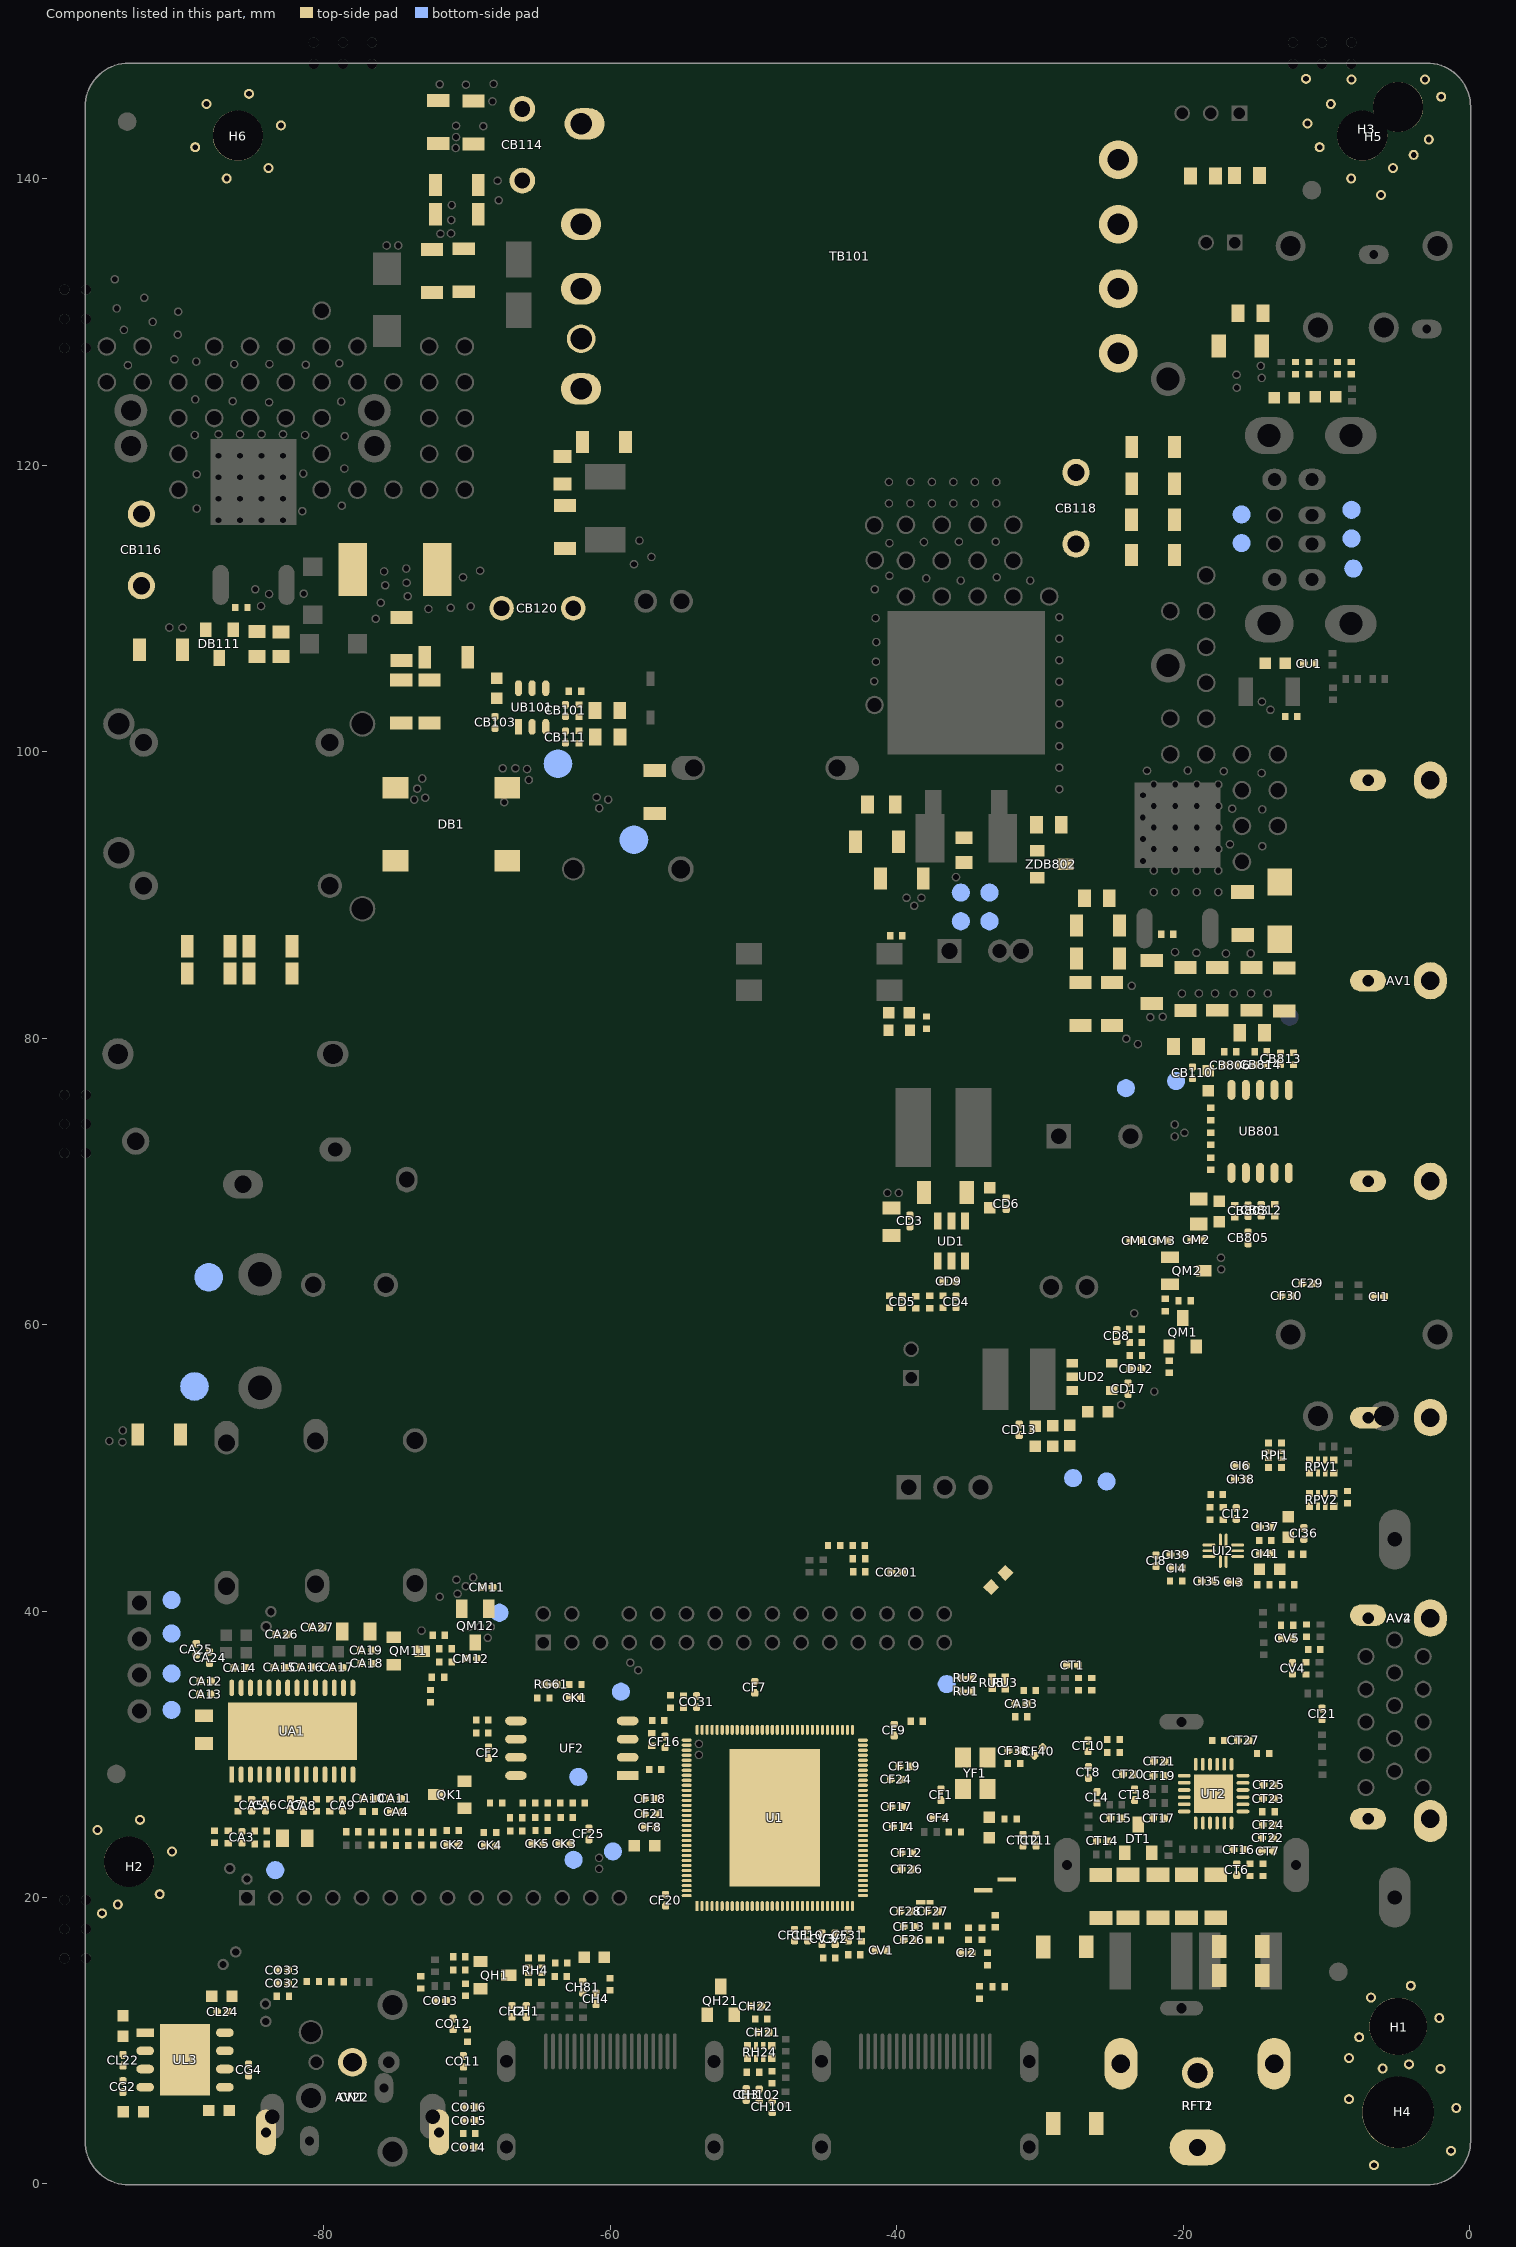
[diagram p0: the components of this part, seen from the top]
# Altium PCB MISC86372.PcbDoc (part 3 of 16)
Units mm, origin at the board's own origin, x right, y up, seen from the top; angles counter-clockwise.
Board outline 96.73 x 148.13 mm, 2 copper layers (TopLayer, BottomLayer), stack 1.571 mm thick; 578 components, 318 nets, 2702 pads, 836 vias.

## Components (designator, comment, footprint, x,y, rotation, side; value= is the part's Value field where it differs from the comment) (continued)
QK1 "General transistor,Dynatron,NPN,0.2A,40V,30-300,SOT-23,MMBT3904(f≥350MHz),BLUE ROCKET" SOT-23 -71.196,27.178 r270 top
QM1 "General transistor,Dynatron,NPN,0.2A,40V,30-300,SOT-23,MMBT3904(f≥350MHz),BLUE ROCKET" SOT-23 -20.041,59.487 r180 top
QM2 "Field-effect transistor,PMOS,-4.2A,-30V,0.052ohm@ID=-4.2A@VGS=-10V,SOT-23-3,AO3401,BLUE ROCKET" SOT-23-1 -19.726,63.762 r90 top
QM11 "General transistor,Dynatron,NPN,0.2A,40V,30-300,SOT-23,MMBT3904(f≥350MHz),BLUE ROCKET" SOT-23 -74.092,37.211 r90 top
QM12 "Field-effect transistor,PMOS,-4.3A,-30V,0.048ohm@ID=-3A@VGS=-4.5V,SOT-23-3L,NCE3407AY,NCEPOWER" SOT-23-1 -69.422,38.957 r0 top
RA1 "4K7ohm-0402-±5%-1/16W" R0402 -87.641,24.236 r270 top
RA2 "4K7ohm-0402-±5%-1/16W" R0402 -86.001,26.458 r270 top
RA3 "1Kohm-0402-±5%-1/16W" R0402 -86.672,24.222 r90 top
RA4 "NC/?" GND#2 -33.96,20.498 r180 top
RA5 "NC/?" GND#2 -32.31,21.262 r180 top
RA8 "NC/100Kohm-0402-±5%-1/16W" R0402 -84.397,24.638 r180 top
RA9 "NC/47Kohm-0402-±5%-1/16W" R0402 -84.397,23.724 r180 top
RA10 "10Kohm-0402-±1%-1/16W" R0402 -80.502,26.448 r90 top
RA11 "15Kohm-0402-±1%-1/16W" R0402 -79.588,26.448 r90 top
RA14 "1Kohm-0402-±5%-1/16W" R0402 -76.849,26.01 r0 top
RA25 "10ohm-0805-±5%-1/8W" R0805 -82.019,24.13 r180 top
RA31 "1Kohm-0402-±5%-1/16W" R0402 -9.235,126.771 r90 top
RA32 "1Kohm-0402-±5%-1/16W" R0402 -12.167,126.771 r90 top
RA33 "Thick-film resistor,RES,1/16W,180ohm,±5%,0402,SMD" R0402 -11.227,126.771 r90 top
RA34 "Thick-film resistor,RES,1/16W,180ohm,±5%,0402,SMD" R0402 -8.27,126.771 r90 top
RA35 "47Kohm-0402-±5%-1/16W" R0402 -31.318,32.614 r180 top
RA36 "10Kohm-0402-±5%-1/16W" R0402 -30.709,34.442 r0 top
RB1 "1M2ohm-1206-±5%-1/4W" R1206 -83.717,84.506 r180 top
RB2 "1M2ohm-1206-±5%-1/4W" R1206 -83.718,86.411 r180 top
RB3 "1M2ohm-1206-±5%-1/4W" R1206 -88.036,86.411 r180 top
RB4 "1M2ohm-1206-±5%-1/4W" R1206 -88.036,84.506 r180 top
RB101 "330Kohm-1206-±5%-1/4W" R1206 -74.6,103.505 r90 top
RB102 "330Kohm-1206-±5%-1/4W" R1206 -74.574,107.848 r270 top
RB103 "Thick-film resistor,RES,1/16W,2Kohm,±1%,0402,SMD" R0402 -62.189,102.845 r90 top
RB104 "NC/47Kohm-0402-±1%-1/16W" R0402 -62.189,101.016 r270 top
RB105 "Thick-film resistor,RES,1/16W,300ohm,±1%,0402,SMD" R0402 -62.465,104.216 r180 top
RB106 "68ohm-0805-±5%-1/8W" R0805 -84.658,107.516 r90 top
RB107 "20ohm-0805-±5%-1/8W" R0805 -82.982,107.49 r90 top
RB109 "10Kohm-0402-±1%-1/16W" R0402 -85.75,110.058 r180 top
RB113 "NC/150Kohm-0805-±1%-1/8W" R0805 -60.182,101.016 r0 top
RB114 "Thick-film resistor,RES,1/4W,10ohm,±5%,1206,SMD" R1206 -60.427,121.615 r0 top
RB117 "10ohm-1206-±5%-1/4W" R1206 -69.545,143.916 r90 top
RB118 "10ohm-1206-±5%-1/4W" R1206 -72.009,143.942 r90 top
RB119 "10ohm-1206-±5%-1/4W" R1206 -91.364,107.112 r180 top
RB120 "NC/10ohm-1206-±5%-1/4W" R1206 -63.17,115.67 r90 top
RB121 "Thick-film resistor,RES,1/8W,30Kohm,±1%,0805,SMD" R0805 -60.208,102.87 r180 top
RB124 "Thick-film resistor,RES,1/4W,47ohm,±5%,1206,SMD" R1206 -22.123,113.716 r180 top
RB125 "Thick-film resistor,RES,1/4W,47ohm,±5%,1206,SMD" R1206 -22.098,121.26 r180 top
RB126 "Thick-film resistor,RES,1/4W,47ohm,±5%,1206,SMD" R1206 -22.098,118.694 r180 top
RB128 "Thick-film resistor,RES,1/4W,47ohm,±5%,1206,SMD" R1206 -39.648,91.135 r0 top
RB129 "Thick-film resistor,RES,1/4W,47ohm,±5%,1206,SMD" R1206 -41.377,93.701 r0 top
RB130 "20ohm-1206-±5%-1/4W" R1206 -56.896,97.18 r90 top
RB131 "Thick-film resistor,RES,1/10W,2Kohm,±1%,0603,SMD" R0603 -39.827,80.543 r0 top
RB132 "Thick-film resistor,RES,1/16W,1.2Kohm,±1%,0402,SMD" R0402 -40.03,87.147 r0 top
RB133 "Thick-film resistor,RES,1/16W,30Kohm,±1%,0402,SMD" R0402 -18.085,74.701 r90 top
RB134 "Thick-film resistor,RES,1/16W,2Kohm,±1%,0402,SMD" R0402 -18.085,72.974 r270 top
RB135 "18Kohm-0402-±1%-1/16W" R0402 -18.085,71.222 r90 top
RB136 "Thick-film resistor,RES,1/4W,47ohm,±5%,1206,SMD" R1206 -22.123,116.18 r180 top
RB139 "NC/Thick-film resistor,RES,1/16W,51ohm,±1%,0402,SMD" R0402 -37.922,81.081 r90 top
RB140 "NC/51Kohm-0805-±1%-1/8W" R0805 -35.306,93.116 r90 top
RB141 "NC/2Mohm-1206-±5%-1/4W" R1206 -72.619,103.505 r270 top
RB142 "NC/2Mohm-1206-±5%-1/4W" R1206 -71.45,106.578 r180 top
RB143 "NC/Thick-film resistor,RES,1/4W,0ohm,±5%,1206,SMD" R1206 -91.491,52.324 r0 top
RB148 "Thick-film resistor,RES,2W,0.36ohm,±5%,2512,SMD" R2512-1 -75.032,112.7 r180 top
RB150 "Thick-film resistor,RES,1/4W,100Kohm,±5%,1206,SMD" R1206 -70.231,133.604 r90 top
RB151 "Thick-film resistor,RES,1/4W,100Kohm,±5%,1206,SMD" R1206 -72.441,133.553 r90 top
RB152 "Thick-film resistor,RES,1/4W,100Kohm,±5%,1206,SMD" R1206 -70.714,139.548 r0 top
RB153 "Thick-film resistor,RES,1/4W,100Kohm,±5%,1206,SMD" R1206 -70.715,137.516 r0 top
RB803 "Thick-film resistor,RES,1/16W,1.3Kohm,±1%,0402,SMD" R0402 -16.713,79.045 r180 top
RB804 "Thick-film resistor,RES,1/16W,20Kohm,±1%,0402,SMD" R0402 -13.614,67.97 r90 top
RB806 "Thick-film resistor,RES,1/16W,100ohm,±5%,0402,SMD" R0402 -16.408,67.92 r90 top
RB807 "Thick-film resistor,RES,1/8W,10ohm,±5%,0805,SMD" R0805 -26.033,89.764 r0 top
RB808 "10Kohm-0402-±1%-1/16W" R0402 -21.107,87.249 r0 top
RB813 "Thick-film resistor,RES,1/16W,100ohm,±5%,0402,SMD" R0402 -12.294,78.562 r270 top
RB814 "Thick-film resistor,RES,1/8W,510Kohm,±1%,0805-Auto,SMD" R0805 -19.812,79.4 r0 top
RB816 "33ohm-0805-±5%-1/8W" R0805 -18.923,67.894 r90 top
RB818 "Thick-film resistor,RES,1/4W,2ohm,±1%,1206,SMD" R1206 -12.954,83.388 r270 top
RB819 "Thick-film resistor,RES,1/4W,2ohm,±1%,1206,SMD" R1206 -17.628,83.439 r270 top
RB820 "Thick-film resistor,RES,1/4W,2ohm,±1%,1206,SMD" R1206 -15.24,83.439 r270 top
RB821 "Thick-film resistor,RES,1/4W,2ohm,±1%,1206,SMD" R1206 -25.959,85.547 r180 top
RB822 "Thick-film resistor,RES,1/4W,2ohm,±1%,1206,SMD" R1206 -25.959,87.859 r180 top
RB823 "Thick-film resistor,RES,1/4W,2ohm,±1%,1206,SMD" R1206 -22.2,83.922 r270 top
RB824 "Thick-film resistor,RES,1/4W,2.4ohm,±5%,1206,SMD" R1206 -19.837,83.414 r270 top
RB825 "Thick-film resistor,RES,1/4W,51Kohm,±1%,1206,SMD" R1206 -24.968,82.372 r270 top
RB826 "Thick-film resistor,RES,1/4W,51Kohm,±1%,1206,SMD" R1206 -27.178,82.372 r270 top
RB833 "Thick-film resistor,RES,1/16W,40.2Kohm,±1%,0402,SMD" R0402 -14.58,79.045 r0 top
RB834 "Thick-film resistor,RES,1/8W,200Kohm,±1%,0805,SMD" R0805 -15.189,80.366 r180 top
RB835 "NC/Thick-film resistor,RES,1/8W,330Kohm,±1%,0805,SMD" R0805 -29.385,94.894 r180 top
RB845 "0ohm-0805-±5%-1/8W" R0805 -18.618,140.183 r0 top
RB846 "NC/0ohm-0805-±5%-1/8W" R0805 -15.545,140.208 r0 top
RB847 "0ohm-0805-±5%-1/8W" R0805 -15.309,130.607 r180 top
RD1 "100Kohm-0402-±5%-1/16W" R0402 -36.779,61.582 r90 top
RD3 "Thick-film resistor,RES,1/16W,33Kohm,±1%,0402,SMD" R0402 -38.677,61.564 r270 top
RD5 "Thick-film resistor,RES,1/16W,6.04Kohm,±1%,0402,SMD" R0402 -40.513,61.589 r90 top
RD6 "NC/?" R0402 -37.694,61.57 r270 top
RD7 "Thick-film resistor,RES,1/16W,100Kohm,±5%,0402,SMD" R0402 -23.333,59.675 r0 top
RD8 "Thick-film resistor,RES,1/16W,13Kohm,±1%,0402,SMD" R0402 -23.317,58.75 r0 top
RD9 "Thick-film resistor,RES,1/16W,12Kohm,±1%,0402,SMD" R0402 -23.305,57.83 r180 top
RF3 "NC/4K7ohm-0402-±5%-1/16W" R0402 -56.865,28.931 r180 top
RF8 "NC/4K7ohm-0402-±5%-1/16W" R0402 -42.647,44.564 r180 top
RF9 "NC/4K7ohm-0402-±5%-1/16W" R0402 -44.374,44.564 r0 top
RF10 "NC/100ohm-0402-±5%-1/16W" R0402 -42.639,43.649 r0 top
RF11 "NC/100ohm-0402-±5%-1/16W" R0402 -42.621,42.739 r0 top
RF12 "68ohm-0402-±5%-1/16W" R0402 -37.338,17.043 r0 top
RF13 "4K7ohm-0402-±5%-1/16W" R0402 -62.433,34.87 r0 top
RF16 "68ohm-0402-±5%-1/16W" R0402 -42.469,17.374 r90 top
RF23 "4K7ohm-0402-±5%-1/16W" R0402 -57.099,31.029 r90 top
RF24 "1Kohm-0402-±5%-1/16W" R0402 -31.814,29.352 r180 top
RF29 "4K7ohm-0402-±5%-1/16W" R0402 -56.642,32.36 r180 top
RF43 "4K7ohm-0402-±5%-1/16W" R0402 -27.305,34.9 r270 top
RF44 "4K7ohm-0402-±5%-1/16W" R0402 -26.391,34.9 r270 top
RFT1 "NC/RF jack,RF JACK,H,IEC,T14.5,CH6.3,12.4×13.2×7.7mm,DIP,LHD-020 assembly,LHD" ANT-IEC14.5-H-4 -19,2.3 r0 top locked
RFT2 "RF jack,RF JACK,H,F,T14.5,CH6.3,without pipe,12.4×13.2×7.7mm,DIP,LHD" T-13.2×12.4×7.7-F14.5 -19,2.3 r0 top locked
RG61 "NC/" R0402SC -64.135,34.87 r180 top
RH3 "1Kohm-0402-±5%-1/16W" R0402 -70.104,13.564 r270 top
RH4 "Resistor array,RES ARRAY,1/16W,4×10Kohm,±5%,0402,SMD" RA0402 -65.253,14.935 r0 top
RH5 "33ohm-0402-±5%-1/16W" R0402 -63.43,15.418 r0 top
RH6 "33ohm-0402-±5%-1/16W" R0402 -63.449,14.494 r0 top
RH23 "1Kohm-0402-±5%-1/16W" R0402 -49.463,11.527 r180 top
RH24 "Resistor array,RES ARRAY,1/16W,4×10Kohm,±5%,0402,SMD" RA0402 -49.58,9.199 r90 top
RH25 "33ohm-0402-±5%-1/16W" R0402 -50.038,7.798 r180 top
RH26 "33ohm-0402-±5%-1/16W" R0402 -48.717,7.442 r270 top
RH81 "22Kohm-0402-±5%-1/16W" R0402 -70.536,14.935 r0 top
RH82 "33Kohm-0402-±5%-1/16W" R0402 -70.536,15.861 r0 top
RH83 "100ohm-0402-±5%-1/16W" R0402 -60.02,13.938 r270 top
RH102 "Thick-film resistor,RES,1/16W,1.2Kohm,±1%,0402,SMD" R0402 -63.043,25.578 r0 top
RH103 "220ohm-0402-±5%-1/16W" R0402 -63.932,26.594 r180 top
RH104 "4K7ohm-0402-±5%-1/16W" R0402 -68.936,31.487 r0 top
RH105 "220ohm-0402-±5%-1/16W" R0402 -62.205,26.594 r180 top
RH106 "4K7ohm-0402-±5%-1/16W" R0402 -68.936,32.401 r0 top
RI1 "75ohm-0402-±5%-1/16W" R0402 -33.122,18.339 r90 top
RI2 "33ohm-0402-±5%-1/16W" R0402 -35,17.478 r90 top
RI3 "NC/1Kohm-0402-±5%-1/16W" R0402 -20.498,42.088 r0 top
RI4 "0ohm-0402-±5%-1/16W" R0402 -8.534,47.955 r90 top
RI5 "NC/0ohm-0402-±5%-1/16W" R0402 -16.472,41.993 r180 top
RI6 "NC/0ohm-0402-±5%-1/16W" R0402 -20.496,42.996 r180 top
RI37 "NC/200Kohm-0402-±5%-1/16W" R0402 -14.275,44.929 r0 top
RI38 "NC/200Kohm-0402-±5%-1/16W" R0402 -17.213,46.805 r90 top
RI39 "NC/200Kohm-0402-±5%-1/16W" R0402 -17.653,48.133 r180 top
RI40 "NC/200Kohm-0402-±5%-1/16W" R0402 -18.127,46.805 r90 top
RI42 "NC/1Kohm-0402-±5%-1/16W" R0402 -12.675,41.834 r0 top
RI43 "NC/1Kohm-0402-±5%-1/16W" R0402 -12.04,43.967 r0 top
RI48 "NC/100ohm-0402-±5%-1/16W" R0402 -14.402,41.834 r0 top
RK1 "4K7ohm-0402-±5%-1/16W" R0402 -67.97,26.594 r180 top
RK2 "1Kohm-0402-±5%-1/16W" R0402 -64.668,33.925 r0 top
RK3 "4K7ohm-0402-±1%-1/16W" R0402 -66.575,25.569 r180 top
RK4 "1Kohm-0402-±5%-1/16W" R0402 -64.808,25.585 r180 top
RK5 "22ohm-0402-±5%-1/16W" R0402 -70.993,24.669 r0 top
RK6 "510ohm-0402-±1%-1/16W" R0402 -78.008,24.595 r0 top
RK7 "680ohm-0402-±1%-1/16W" R0402 -72.782,23.663 r0 top
RK8 "1Kohm-0402-±1%-1/16W" R0402 -72.791,24.559 r0 top
RK9 "1K2ohm-0402-±1%-1/16W" R0402 -74.535,24.567 r0 top
RK10 "1Kohm-0402-±5%-1/16W" R0402 -68.395,24.544 r180 top
RK11 "2K2ohm-0402-±1%-1/16W" R0402 -74.534,23.641 r0 top
RK12 "4K7ohm-0402-±1%-1/16W" R0402 -76.246,23.658 r0 top
RK13 "33Kohm-0402-±5%-1/16W" R0402 -65.679,26.594 r180 top
RK14 "510ohm-0402-±1%-1/16W" R0402 -64.795,24.666 r0 top
RK15 "10Kohm-0402-±5%-1/16W" R0402 -66.573,24.648 r0 top
RK16 "15Kohm-0402-±1%-1/16W" R0402 -76.275,24.573 r0 top
RM1 "10Kohm-0402-±5%-1/16W" R0402 -38.608,32.309 r180 top
RM2 "4K7ohm-0402-±5%-1/16W" R0402 -20.98,57.048 r90 top
RM3 "4K7ohm-0402-±5%-1/16W" R0402 -21.252,61.366 r90 top
RM4 "Thick-film resistor,RES,1/16W,100Kohm,±5%,0402,SMD" R0402 -19.906,61.663 r180 top
RM11 "4K7ohm-0402-±5%-1/16W" R0402 -72.028,35.377 r180 top
RM12 "10Kohm-0402-±5%-1/16W" R0402 -72.542,34.061 r270 top
RM13 "4K7ohm-0402-±5%-1/16W" R0402 -71.975,38.303 r180 top
RM14 "47Kohm-0402-±5%-1/16W" R0402 -71.501,36.452 r0 top
RM15 "NC/4K7ohm-0402-±5%-1/16W" R0402 -71.501,37.363 r180 top
RO1 "NC/75ohm-0402-±5%-1/16W" R0402 -36.855,18.009 r180 top
RO2 "NC/0ohm-0402-±5%-1/16W" R0402 -73.228,14.072 r90 top
RO3 "NC/0ohm-0402-±5%-1/16W" R0402 -80.762,14.129 r0 top
RO4 "NC/0ohm-0402-±5%-1/16W" R0402 -79.045,14.118 r180 top
RO12 "NC/510ohm-0402-±1%-1/16W" R0402 -69.977,10.363 r270 top
RO15 "NC/510ohm-0402-±1%-1/16W" R0402 -69.85,3.516 r0 top
RO21 "Thick-film resistor,RES,1/16W,150ohm,±1%,0402,SMD" R0402 -54.89,33.674 r270 top
RO22 "75ohm-0402-±5%-1/16W" R0402 -55.804,33.68 r270 top
RO33 "NC/0ohm-0402-±5%-1/16W" R0402 -82.855,13.106 r0 top
ROUT+ "DM0" TP -90.627,40.767 r180 bottom
ROUT- "DM0" TP -90.627,38.43 r180 bottom
RPI1 "Resistor array,RES ARRAY,1/16W,4×10Kohm,±5%,0402,SMD" RA0402 -13.589,50.876 r180 top
RPV1 "NC/Resistor array,RES ARRAY,1/16W,4×10Kohm,±5%,0402,SMD" RA0402 -10.342,50.082 r270 top
RPV2 "NC/Resistor array,RES ARRAY,1/16W,4×10Kohm,±5%,0402,SMD" RA0402 -10.342,47.759 r90 top
RT1 "Ferrite bead,BEAD,300ohm,0402,800mA,SMD,TP,FCM1005KF-301T08" R0402 -35.941,24.566 r180 top
RT2 "22ohm-0402-±5%-1/16W" R0402 -15.345,21.924 r90 top
RT3 "22ohm-0402-±5%-1/16W" R0402 -14.43,21.924 r90 top
RT4 "0ohm-0402-±5%-1/16W" R0402 -24.867,30.124 r180 top
RT5 "0ohm-0402-±5%-1/16W" R0402 -24.867,31.039 r180 top
RT6 "1K8ohm-0402-±5%-1/16W" R0402 -14.049,25.988 r180 top
RT7 "10Kohm-0402-±5%-1/16W" R0402 -32.055,25.476 r0 top
RT8 "100ohm-0402-±5%-1/16W" R0402 -17.551,30.963 r180 top
RU1 "NC/0ohm-0402-PCB" R0402SC -35.149,34.413 r0 top
RU2 "NC/0ohm-0402-PCB" R0402SC -35.149,35.327 r0 top
RU3 "NC/0ohm-0402-PCB" R0402SC -32.423,34.976 r90 top
RU4 "0ohm-0402-±5%-1/16W" R0402 -12.464,102.457 r180 top
RU5 "NC/0ohm-0402-PCB" R0402SC -33.335,34.99 r90 top
RV1 "75ohm-0402-±5%-1/16W" R0402 -34.043,17.478 r270 top
RV2 "33ohm-0402-±5%-1/16W" R0402 -33.655,15.705 r270 top
RV3 "75ohm-0402-±5%-1/16W" R0402 -32.893,13.767 r180 top
RV4 "33ohm-0402-±5%-1/16W" R0402 -42.977,16.002 r180 top
RV5 "75ohm-0402-±5%-1/16W" R0402 -34.214,13.368 r90 top
RV6 "NC/10Kohm-0402-±5%-1/16W" R0402 -11.43,35.992 r90 top
RV7 "NC/100ohm-0402-±5%-1/16W" R0402 -10.846,37.313 r180 top
RV8 "NC/10Kohm-0402-±5%-1/16W" R0402 -11.396,38.633 r90 top
RV9 "NC/100ohm-0402-±5%-1/16W" R0402 -12.751,39.012 r180 top
RV10 "33ohm-0402-±5%-1/16W" R0402 -44.704,15.773 r180 top
RXD "" TP -62.23,28.423 r90 bottom
S/N1 "Barcode" Barcode -17.704,58.953 r270 bottom
TB101 "Transformer,EQ2414,300uH,0.2×1P,26Ts,H14.5MAX,SYEQ2414Z-T012064B(BLACK),DIP,SQ" T/EQ2414*10 -40.538,134.569 r0 top
TP-TDT "" TP-TDT -61,96.5 r135 bottom
TP_12VA+ "NC/" TP -35.527,90.154 r180 bottom
TP_12VA- "NC/" TP -33.527,90.154 r180 bottom
TP_12VB+ "NC/" TP -35.527,88.154 r180 bottom
TP_12VB- "NC/" TP -33.527,88.154 r180 bottom
TP_L "NC/" TP-80 -88.036,63.297 r180 bottom
TP_LED+ "NC/" TP -20.5,77 r180 bottom
TP_LED- "NC/" TP -24,76.5 r180 bottom
TP_N "NC/" TP-80 -89.027,55.677 r180 bottom
TXD "" TP -62.56,22.631 r180 bottom
U1 "TV main chip,IC Main Chip,MSD3553ZW-005X,32bit,Single-Core,QFN128,SMD,MTK" QFN128/0.35-1-9 -48.513,25.556 r90 top locked
UA1 "Audio amplifier,IC Audio AMP,Class D,2×10W@13.0V@8ohm,HTSSOP-28,SMD,RDA3118E28B,RDA" SSOP28/0.65-5 -82.197,31.611 r90 top
UART_RX "DM0" TP -27.686,49.276 r90 bottom
UART_TX "DM0" TP -25.349,49.047 r90 bottom
UB101 "PWM controller,IC PWM Controller,100KHZ,SOT23-6,SMD,LD5537B3GL,Leadtrend" SOT-26 -65.456,103.077 r180 top
UB801 "PWM controller,IC PWM Controller,10KHz-1MHz,SSOP10,SMD,SY7710FHC,silergy" SOP10/1.0-1 -14.63,73.482 r90 top
UD1 "DC-DC converter,IC DCDC,Syn,2A,18V,500KHz,SOT23-6,SMD,LC2332CB6TR,Leadchip" SOT-23-6 -36.189,65.831 r180 top
UD2 "DC-DC converter,IC DCDC,Syn,1.2A,6.0V,1.5MHz,SOT23-5,SMD,TMI3408,TOLL" SOT-23-5 -26.365,56.343 r270 top locked
UF2 "SPI FLASH chip,IC SPI FLASH,4MB,32Mb,SOIC8,SMD,W25Q32JVSSIQ,Winbond" SOIC8 -62.687,30.42 r180 top locked
UI2 "NC/AZAW2213F" QFN10/0.4 -17.206,44.208 r270 top
UL3 "LDO regulator,IC LDO,1A,3.3V,12V,ESOP-8,SMD,LC1118CS8TR1833,Leadchip" SOP8/1.27-3 -89.689,8.66 r0 top
UT2 "Silicon RF tuner,IC Si Tuner,QFN24,SMD,R842,Rafael" QFN24/0.5-3 -17.882,27.254 r90 top
VCC_PANEL "TEST" TP -67.742,39.878 r270 bottom
VDDC_CORE "TEST" TP -36.513,34.9 r0 bottom
XXXXXX "PCB_TIME" PCB_TIME -19.845,45.677 r180 top
XXXXXXXXXXXXXX "PCB_NAME" PCB_NAME -18.721,38.285 r180 top
YF1 "Passive crystal,SPXO,24MHz,±10ppm,12pF,SMD3225,SMD,2.3.3.240001234,MDH" XTAL-S-3 -34.519,28.677 r270 top
ZDB801 "TVS diode,DIO ESD,121V,SMA,SMD,SMAJ75A,YJ" DIODE-SMA-1 -13.259,88.9 r90 top
ZDB802 "Zener diode,DIO ZEN,5.6V,350mW,SOT-23,SMD,BZX84C5V6,KEXIN" SO-23 -29.185,92.138 r90 top
用于U1 "NC/Glue, 0.1g, silicone" "Heat-Shrinkable Tube" -44.936,29.365 r90 top

## Footprints (in the part's own frame and the unit in brackets; to place one, negate y for a bottom-side part, rotate by r counter-clockwise, add the part's x,y. Pads: shape width x height; smd on the part's side, far side on the other; paste and mask are expansions set on the pad)
AI_GRIPPER_V [mm] "3D shape for vertical type AI equipment  (AI爪子)"
  round 1.5 on Mech5: 0(0,-2.5) 1(0,0) 2(0,2.5)
  body extent -29.13,-4.7 2.5,4.7, height 54.74
ANT-IEC14.5-H-4 [mm] "联宏达；13.2×12.4×7.7mm LHD-020 中心高度6.3mm 160323(18.03.09更新脚距）,向内扩宽丝印,0703_2018（18.08.29 更新短槽孔）"
  oval 2.5x3.8 on Top Overlay paste-4 mask-4: 0(-5.35,6.1) 0(5.35,6.1)
  oval 4.1x2.7 on Top Overlay paste-4 mask-4: 0(0,0.25)
  round 2.4 on Top Overlay: 0(0,5.45)
  round 2.2 hole 1.4: 1(0,5.45)
  oval 2.3x3.6 hole 1.3 slot 2.6 at 90 deg: 2(-5.35,6.1) 4(5.35,6.1)
  oval 3.9x2.5 hole 1.2 slot 2.6 at 0 deg: 3(0,0.25)
  KeepOutLayer pour cut-out: 0,3.95 -0.574,4.064 -1.061,4.389 -1.386,4.876 -1.5,5.45 -1.5,5.45 -1.386,6.024 -1.061,6.511 -0.574,6.836 0,6.95 0,6.95 0.574,6.836 1.061,6.511 1.386,6.024 1.5,5.45 1.5,5.45 1.386,4.876 1.061,4.389 0.574,4.064 0,3.95
  silkscreen extent -6.3,0 6.3,7.9, body extent -7.55,-35.2 7.55,7.7, height 13.76
ASSE3.5C-3#1 [mm] "定位孔(顶底层上锡) (18.11.28 切换为扇形paste）"
  round 3.5 hole 3.5 unplated mask+0: 0(0,0)
  round 0.7 hole 0.4: 1(-0.778,-2.994) 2(-1.881,-3.602) 3(-2.195,2.213) 4(0.774,2.919) 5(3.005,0.716) 6(2.143,-2.266)
  KeepOutLayer pour cut-out: 0,-2.05 -0.785,-1.894 -1.45,-1.45 -1.894,-0.785 -2.05,0 -2.05,0 -1.894,0.785 -1.45,1.45 -0.785,1.894 0,2.05 0,2.05 0.785,1.894 1.45,1.45 1.894,0.785 2.05,0 2.05,0 1.894,-0.785 1.45,-1.45 0.785,-1.894 0,-2.05
ASSE3.5C-3#2 [mm] "定位孔(顶底层上锡) (18.11.28 切换为扇形paste）"
  round 3.5 hole 3.5 unplated mask+0: 0(0,0)
  round 0.7 hole 0.4: 1(-0.778,-2.994) 2(-2.979,-0.807) 3(-2.195,2.213) 4(-0.757,3.914) 5(3.588,-1.344) 6(2.143,-2.266)
  KeepOutLayer pour cut-out: 0,-2.05 -0.785,-1.894 -1.45,-1.45 -1.894,-0.785 -2.05,0 -2.05,0 -1.894,0.785 -1.45,1.45 -0.785,1.894 0,2.05 0,2.05 0.785,1.894 1.45,1.45 1.894,0.785 2.05,0 2.05,0 1.894,-0.785 1.45,-1.45 0.785,-1.894 0,-2.05
ASSE3.5C-3#3 [mm] "定位孔(顶底层上锡) (18.11.28 切换为扇形paste）"
  round 3.5 hole 3.5 unplated mask+0: 0(0,0)
  round 0.7 hole 0.4: 1(-1.198,-6.138) 2(-6.331,-1.156) 3(-6.43,1.964) 4(1.876,1.914) 5(3.005,0.716) 6(2.143,-2.266)
  KeepOutLayer pour cut-out: 0,-2.05 -0.785,-1.894 -1.45,-1.45 -1.894,-0.785 -2.05,0 -2.05,0 -1.894,0.785 -1.45,1.45 -0.785,1.894 0,2.05 0,2.05 0.785,1.894 1.45,1.45 1.894,0.785 2.05,0 2.05,0 1.894,-0.785 1.45,-1.45 0.785,-1.894 0,-2.05
ASSE3.5C-3#4 [mm] "定位孔(顶底层上锡) (18.11.28 切换为扇形paste）"
  round 3.5 hole 3.5 unplated mask+0: 0(0,0)
  round 0.7 hole 0.4: 1(-0.778,-2.994) 2(-2.979,-0.807) 3(-2.195,2.213) 4(0.774,2.919) 5(3.005,0.716) 6(2.143,-2.266)
  KeepOutLayer pour cut-out: 0,-2.05 -0.785,-1.894 -1.45,-1.45 -1.894,-0.785 -2.05,0 -2.05,0 -1.894,0.785 -1.45,1.45 -0.785,1.894 0,2.05 0,2.05 0.785,1.894 1.45,1.45 1.894,0.785 2.05,0 2.05,0 1.894,-0.785 1.45,-1.45 0.785,-1.894 0,-2.05
ASSE4.0C-3 [mm] "定位孔(顶底层上锡)(17.12.09更新过孔位置）18.11.22 更新paste形状为扇形。"
  round 4 hole 4 unplated mask+0: 0(0,0)
  round 0.7 hole 0.4: 1(-2.72,-0.754) 2(-1.893,2.011) 3(0.891,2.84) 4(2.873,0.584) 5(0.758,-2.643) 6(-1.075,-2.937)
  KeepOutLayer pour cut-out: 0,-2.3 -0.88,-2.125 -1.626,-1.626 -2.125,-0.88 -2.3,0 -2.3,0 -2.125,0.88 -1.626,1.626 -0.88,2.125 0,2.3 0,2.3 0.88,2.125 1.626,1.626 2.125,0.88 2.3,0 2.3,0 2.125,-0.88 1.626,-1.626 0.88,-2.125 0,-2.3
ASSE5.0C-3 [mm] "定位孔(顶底层上锡) (18.12.13更新）"
  round 5 hole 5 unplated mask+0: 0(0,0)
  round 0.7 hole 0.4: 1(-3.423,3.787) 2(-3.432,0.923) 3(-1.678,-3.689) 4(3.691,-2.689) 5(4.06,0.309) 6(2.958,3.038)
  KeepOutLayer pour cut-out: 0,-2.8 -1.072,-2.587 -1.98,-1.98 -2.587,-1.072 -2.8,0 -2.8,0 -2.587,1.072 -1.98,1.98 -1.072,2.587 0,2.8 0,2.8 1.072,2.587 1.98,1.98 2.587,1.072 2.8,0 2.8,0 2.587,-1.072 1.98,-1.98 1.072,-2.587 0,-2.8
AV1-H-4 [mm] "强生；AV38A-01S-5020;中心高度为5.5mm;14.08.09;170502更新信号脚孔径;170902更新接地脚宽度,17.12.29更新接地脚孔长度（18.05.07 更新地脚孔长?"
  round 2 hole 1.3 mask+0.076: 1(0,8.05)
  round 2.2 on Top Overlay mask+0.076: 2(0,8.05)
  oval 1.4x3.2 hole 0.7 slot 2.5 at 90 deg mask+0.076: 2(6.05,3.15) 3(-6.05,3.15)
  oval 1.6x3.4 on Top Overlay mask+0.076: 3(-6.05,3.15) 3(6.05,3.15)
  silkscreen extent -6.4,0 6.4,8.7, body extent -7.25,-51.37 7.25,8.55, height 12.75
AV3-H14-15#1 [mm] "宇球；RC075-F03L3BY-A; 中心高度：5.5mm;15.11.24;170401兼容物料，更新高度;170802加大接地脚焊盘（18.03.09更新孔距）"
  oval 2.8x2.5 on Top Overlay: 0(-14,2.75) 0(0,2.75) 0(14,2.75)
  oval 1.7x2.7 on Top Overlay: 0(-14,7.1) 0(0,7.1) 0(14,7.1)
  oval 1.5x2.5 hole 0.8 slot 1.8 at 90 deg: 1(-14,7.1) 3(0,7.1) 5(14,7.1)
  oval 2.6x2.3 hole 1.3 slot 1.6 at 0 deg: 2(-14,2.75) 4(0,2.75) 6(14,2.75)
  silkscreen extent -20.3,0 20.3,7.8, body extent -20.1,-9 20.1,7.9, height 10.7
AV3-H14-15#2 [mm] "宇球；RC075-F03L3BY-A; 中心高度：5.5mm;15.11.24;170401兼容物料，更新高度;170802加大接地脚焊盘（18.03.09更新孔距）"
  oval 2.8x2.5 on Top Overlay: 0(-14,2.75) 0(0,2.75) 0(14,2.75)
  oval 1.7x2.7 on Top Overlay: 0(-14,7.1) 0(0,7.1) 0(14,7.1)
  oval 1.5x2.5 hole 0.8 slot 1.8 at 90 deg: 1(-14,7.1) 5(14,7.1)
  oval 2.6x2.3 hole 1.3 slot 1.6 at 0 deg: 2(-14,2.75) 4(0,2.75) 6(14,2.75)
  oval 1.5x2.5 hole 0.8 slot 1.8 at 90 deg copper offset 0.2,0: 3(0,7.1)
  silkscreen extent -20.3,0 20.3,7.8, body extent -20.1,-9 20.1,7.9, height 10.7
AV3-H14-15#3 [mm] "宇球；RC075-F03L3BY-A; 中心高度：5.5mm;15.11.24;170401兼容物料，更新高度;170802加大接地脚焊盘（18.03.09更新孔距）"
  oval 2.8x2.5 on Top Overlay: 0(-14,2.75) 0(0,2.75) 0(14,2.75)
  oval 1.7x2.7 on Top Overlay: 0(-14,7.1) 0(0,7.1) 0(14,7.1)
  oval 1.5x2.5 hole 0.8 slot 1.8 at 90 deg: 1(-14,7.1) 5(14,7.1)
  oval 2.6x2.3 hole 1.3 slot 1.6 at 0 deg copper offset -0.32,0: 2(-14,2.75)
  oval 1.5x2.5 hole 0.8 slot 1.8 at 90 deg copper offset 0.2,0: 3(0,7.1)
  oval 2.6x2.3 hole 1.3 slot 1.6 at 0 deg: 4(0,2.75) 6(14,2.75)
  silkscreen extent -20.3,0 20.3,7.8, body extent -20.1,-9 20.1,7.9, height 10.7
B/YBS3010A [mm] "YJ,YBS3010A,18.04.17"
  rect 1.5x1.8 smd: 1(2.55,3.9) 2(2.55,-3.9) 3(-2.55,-3.9) 4(-2.55,3.9)
  silkscreen extent -3.35,-3.7 3.35,5.74, body extent -3.35,-3.7 3.35,3.7, height 1.5
Barcode [mm] "(18.12.17 更新为白油）"
  round 0.3 on Mech2: 0(0,0)
  silkscreen extent -15,-4 15,4
C0402 [mm] "片式电容  2018.10.7 替换为兼容0201封装"
  rrect50% 0.45x0.5 smd mask+0.051: 1(-0.425,0) 2(0.425,0)
  rect 0.3x0.3 smd mask+0.051: 1(-0.25,0) 2(0.25,0)
  rect 0.6x0.6 on Top Solder: 2(0,0)
  TopLayer pour cut-out: -0.318,0.302 -0.318,-0.303 0.306,-0.303 0.306,0.302
  silkscreen extent -0.88,-0.4 0.88,0.4, body extent -0.5,-0.25 0.5,0.25, height 0.5
C0603 [mm] "片式电容"
  rect 0.8x0.8 smd mask+0.076: 1(-0.706,0) 2(0.706,0)
  silkscreen extent -1.39,-0.55 1.39,0.55, body extent -0.8,-0.4 0.8,0.4, height 0.8
C0805 [mm] "片式电容"
  rect 0.9x1.25 smd mask+0.076: 1(-0.966,0) 2(0.966,0)
  silkscreen extent -1.73,-0.78 1.73,0.78, body extent -1,-0.62 1,0.63, height 1.25
C1206 [mm] "片式电容"
  rect 1x1.6 smd mask+0.076: 1(-1.5,-0.001) 2(1.5,0.001)
  silkscreen extent -2.39,-0.95 2.39,0.95, body extent -1.6,-0.8 1.6,0.8, height 1.3
CAP7.5*5-V-5-1 [mm] "TDK，CC45SL3DD101JYSNA，外K型引脚，AI，0713_2018"
  round 2.1 on Top Overlay: 0(-2.5,0) 0(2.5,0)
  round 1.9 hole 1.2 mask+0.051: 1(-2.5,0) 2(2.5,0)
  BottomLayer lines w0.6: 2.19,-0.39 4.056,-1.556 ; -2.89,-0.31 -4.056,1.556 ; 2.5,0 4.056,-1.556 ; -2.5,0 -4.056,1.556 ; 2.89,0.31 4.056,-1.556 ; -2.19,0.39 -4.056,1.556
  silkscreen extent -5.5,-2.5 5.5,2.5
CAP8*2.5-V-5 [mm] "C242G472J20A201(编带/法拉)"
  round 1.8 hole 1.1: 1(-2.5,0) 2(2.5,0)
  round 2 on Top Overlay: 1(-2.5,0) 1(2.5,0)
  BottomLayer lines w0.6: -2.15,0.456 -2.215,0.493 -4.056,1.556 ; 2.956,0.35 2.993,0.285 4.056,-1.556 ; -2.5,0 -2.627,0.127 -2.678,0.178 -2.856,0.356 -3.008,0.508 -3.033,0.533 -3.084,0.584 -3.11,0.61 -4.056,1.556 ; 2.5,0 4.056,-1.556 ; -2.956,-0.35 -2.993,-0.285 ; 2.15,-0.456 2.215,-0.493 4.056,-1.556 ; -4.056,1.556 -3.509,0.61 -3.495,0.584 -3.465,0.533 -3.363,0.356 -3.334,0.306 -2.993,-0.285 ; -2.993,-0.285 -2.993,-0.285
  silkscreen extent -4,-1.25 4,1.25
CAP8.5*5-V-5 [mm] "TDK，CC45SL3AD221JYSNA，外K型引脚，AI，0713_2018"
  round 2.1 on Top Overlay: 0(-2.5,0) 0(2.5,0)
  round 1.9 hole 1.2 mask+0.051: 1(-2.5,0) 2(2.5,0)
  BottomLayer lines w0.6: 2.19,-0.39 4.056,-1.556 ; -2.89,-0.31 -2.92,-0.262 -4.056,1.556 ; 2.5,0 4.056,-1.556 ; -2.5,0 -4.056,1.556 ; 2.89,0.31 4.056,-1.556 ; -2.19,0.39 -2.238,0.42 -4.056,1.556
  silkscreen extent -5.5,-2.5 5.5,2.5
CAP10*4.5-V-5 [mm] "YU102472M090DAND5H，陶瓷电容，17.12.22"
  round 1.7 hole 1.1: 1(-2.5,0) 2(2.5,0)
  round 1.9 on Top Overlay: 41(2.5,0) 42(-2.5,0)
  BottomLayer lines w0.6: -2.89,-0.31 -4.056,1.556 ; -2.5,0 -4.056,1.556 ; -2.19,0.39 -4.056,1.556 ; 2.19,-0.39 4.056,-1.556 ; 2.5,0 4.056,-1.556 ; 2.89,0.31 4.056,-1.556
  silkscreen extent -5.55,-2.25 5.55,2.25